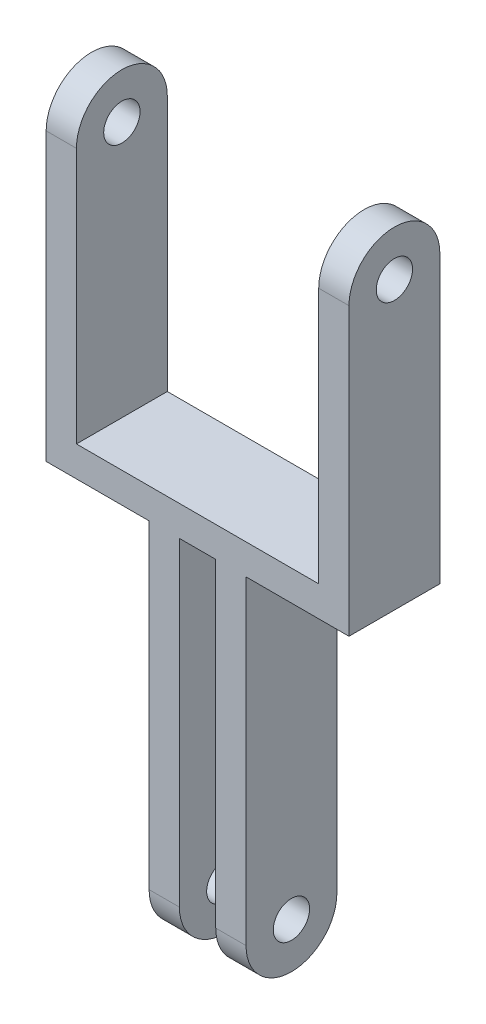
SolidWorks part; units mm, degrees
ref_plane "Front Plane" through (0, 0, 0) normal (0, 0, 1) x (1, 0, 0)
ref_plane "Top Plane" through (0, 0, 0) normal (0, 1, 0) x (1, 0, 0)
ref_plane "Right Plane" through (0, 0, 0) normal (1, 0, 0) x (0, 0, -1)
other "Configuration Table"
sketch "Sketch1" plane through (0, 0, 0) normal (0, 0, 1) x (1, 0, 0)
  line L0 (0, 0) -> (0, 164.9526) construction
  line L1 (-3, 0) -> (-3, 65)
  line L2 (-3, 65) -> (3, 65)
  line L4 (20, 70) -> (-20, 70)
  line L5 (-20, 70) -> (-20, 120)
  line L6 (-20, 120) -> (-25, 120)
  line L7 (-25, 120) -> (-25, 65)
  line L8 (-25, 65) -> (-8, 65)
  line L9 (-8, 65) -> (-8, 0)
  line L10 (-8, 0) -> (-3, 0)
  line L11 (8, 0) -> (3, 0)
  line L12 (8, 65) -> (8, 0)
  line L13 (25, 65) -> (8, 65)
  line L14 (25, 120) -> (25, 65)
  line L15 (20, 120) -> (25, 120)
  line L16 (20, 70) -> (20, 120)
  line L17 (3, 0) -> (3, 65)
  point P20 (0, 70)
  point P21 (0, 65)
  dimension "D1" = 120
  dimension "D2" = 6
  dimension "D3" = 16
  dimension "D4" = 40
  dimension "D5" = 50
  dimension "D6" = 5
  dimension "D7" = 50
extrude "Boss-Extrude1" add sketch "Sketch1" along normal blind 15
sketch "Sketch2" plane through (-25, 0, 0) normal (-1, 0, 0) x (0, 0, 1)
  line L0 (0, 112.2719) -> (-22.4268, 115.8847)
  line L1 (-22.4268, 115.8847) -> (0, 149.1264)
  line L2 (0, 149.1264) -> (35.6198, 129.7213)
  line L3 (35.6198, 129.7213) -> (15, 112.2719)
  line L4 (0, 12.2719) -> (-15.3016, 4.7719)
  line L5 (-15.3016, 4.7719) -> (-3.2806, -11.4276)
  line L6 (-3.2806, -11.4276) -> (32.4691, -8.1872)
  line L7 (32.4691, -8.1872) -> (24.8383, 8.5219)
  line L8 (24.8383, 8.5219) -> (15, 12.2719)
  circle A0 centre (7.5, 112.2719) radius 3
  circle A1 centre (7.5, 12.2719) radius 3
  arc A2 (15, 112.2719) -> (0, 112.2719) centre (7.5, 112.2719) ccw
  arc A3 (0, 12.2719) -> (15, 12.2719) centre (7.5, 12.2719) ccw
  dimension "D1" = 100
  dimension "D2" = 6
  dimension "D3" = 6
extrude "Cut-Extrude1" cut sketch "Sketch2" against normal through all
